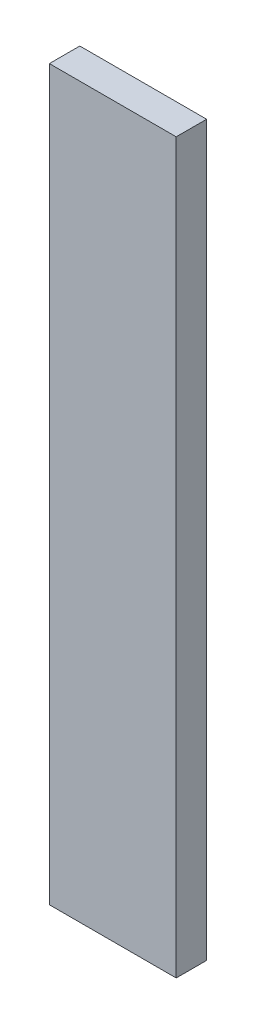
from build123d import *

# Parameters (mm, degrees)
SKETCH1_W           = 125
SKETCH1_H           = 718
BOSS_EXTRUDE1_DEPTH = 30


with BuildPart() as part:
    # Sketch1 → Boss-Extrude1 (new body)
    with BuildSketch(Plane.XY):
        with Locations((62.5, 359)):
            Rectangle(SKETCH1_W, SKETCH1_H)
    extrude(amount=BOSS_EXTRUDE1_DEPTH)


solid = part.part
